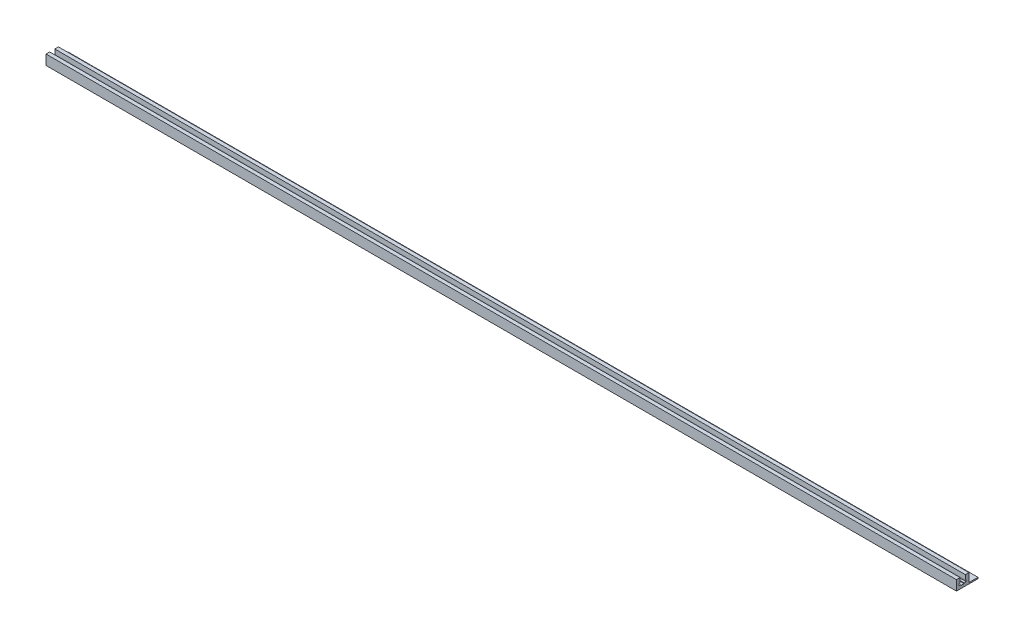
from build123d import *

# Parameters (mm, degrees)
SKETCH_1_W             = 30
SKETCH_1_H             = 24
EXTRUDE_1_DEPTH        = 2200
CUT_EXTRUDE_1_DEPTH    = 2201.083862038
SKETCH_5_W             = 2200
SKETCH_5_H             = 3
EXTRUDE_2_DEPTH        = 22
CUT_EXTRUDE_2_DEPTH    = 22
PATTERN_LINEAR_1_COUNT = 6
PATTERN_LINEAR_1_PITCH = 510


with BuildPart() as part:
    # 草图1 → 凸台-拉伸1 (new body)
    with BuildSketch(Plane(origin=(0, 0, 0), x_dir=(0, 0, -1), z_dir=(1, 0, 0))):
        Rectangle(SKETCH_1_W, SKETCH_1_H)
    extrude(amount=EXTRUDE_1_DEPTH)

    # 草图2 → 切除-拉伸1 (cut, through all)
    with BuildSketch(Plane(origin=(2200, 0, 0), x_dir=(0, 0, -1), z_dir=(1, 0, 0))):
        Polygon((-6.2, 12), (-6.2, 0.7), (-8.5, 0.7), (-8.5, -3.9), (-3.5, -3.9), (-3.5, -5.5), (3.5, -5.5), (3.5, -3.9), (8.5, -3.9), (8.5, 0.7), (6.2, 0.7), (6.2, 12), align=None)
    extrude(amount=-CUT_EXTRUDE_1_DEPTH, mode=Mode.SUBTRACT)

    # 草图5 → 凸台-拉伸2 (add)
    with BuildSketch(Plane(origin=(0, 0, -15), x_dir=(-1, 0, 0), z_dir=(0, 0, -1))):
        with Locations((-1100, -10.5)):
            Rectangle(SKETCH_5_W, SKETCH_5_H)
    extrude(amount=EXTRUDE_2_DEPTH)

    # 草图6 → 切除-拉伸2 (cut)
    with BuildSketch(Plane.XZ.offset(12)):
        with BuildLine():
            Line((33.5, -22), (33.5, -30))
            ThreePointArc((33.5, -30), (30, -33.5), (26.5, -30))
            Line((26.5, -30), (26.5, -22))
            ThreePointArc((26.5, -22), (30, -18.5), (33.5, -22))
        make_face()
    cut_extrude_2 = extrude(amount=-CUT_EXTRUDE_2_DEPTH, mode=Mode.SUBTRACT)

    # 阵列(线性)1: 切除-拉伸2 ×6
    with Locations(*[(i * PATTERN_LINEAR_1_PITCH, 0, 0) for i in range(1, PATTERN_LINEAR_1_COUNT)]):
        add(cut_extrude_2, mode=Mode.SUBTRACT)


solid = part.part
